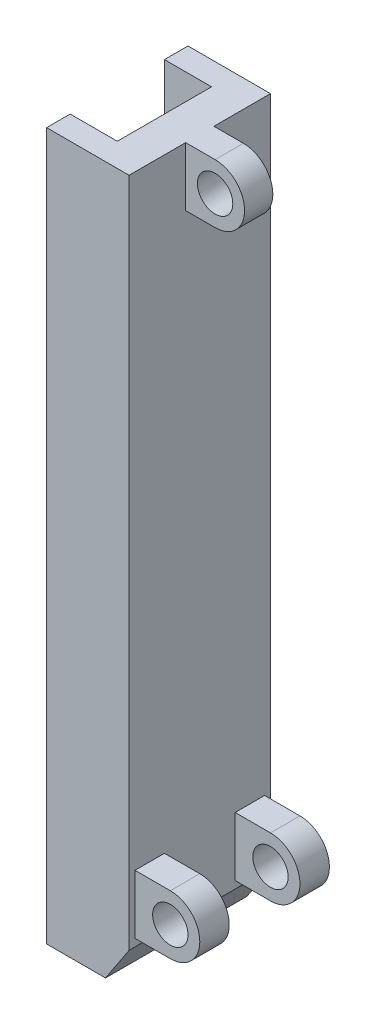
SolidWorks part; units mm, degrees
ref_plane "Front Plane" through (0, 0, 0) normal (0, 0, 1) x (1, 0, 0)
ref_plane "Top Plane" through (0, 0, 0) normal (0, 1, 0) x (1, 0, 0)
ref_plane "Right Plane" through (0, 0, 0) normal (1, 0, 0) x (0, 0, -1)
other "Configuration Table"
sketch "Sketch1" plane through (0, 0, 0) normal (0, 1, 0) x (1, 0, 0)
  line L0 (-20, 40) -> (-20, 60)
  line L1 (-20, 40) -> (20, 40)
  line L3 (-20, -40) -> (20, -40)
  line L4 (20, 40) -> (20, -40)
  line L5 (-20, 40) -> (20, -40) construction
  line L6 (-20, -40) -> (20, 40) construction
  line L7 (-20, 60) -> (50, 60)
  line L9 (-20, -60) -> (50, -60)
  line L10 (50, 60) -> (50, -60)
  line L11 (-50, 60) -> (50, -60) construction
  line L12 (-50, -60) -> (50, 60) construction
  line L13 (-20, -40) -> (-20, -60)
  point P0 (0, 0)
  point P6 (0, 0)
  dimension "D1" = 40
  dimension "D2" = 80
  dimension "D3" = 120
  dimension "D4" = 30
extrude "Boss-Extrude1" add sketch "Sketch1" along normal blind 600
sketch "Sketch2" plane through (0, 0, -60) normal (0, 0, -1) x (-1, 0, 0)
  line L0 (10.0315, 61.6536) -> (-80, 61.6536) construction
  line L1 (-34.9842, 36.6536) -> (-80, 36.6536)
  line L2 (-34.9842, 86.6536) -> (-80, 86.6536)
  line L3 (-50, 600) -> (-50, 0) construction
  line L4 (-34.9842, 86.6536) -> (-34.9842, 36.6536)
  arc A1 (-80, 86.6536) -> (-80, 36.6536) centre (-80, 61.6536) ccw
  circle A2 centre (-80, 61.6536) radius 15
  point P2 (-44.9842, 61.6536)
  dimension "D1" = 25
  dimension "D3" = 30
  dimension "D2" = 30
extrude "Boss-Extrude2" add sketch "Sketch2" against normal blind 30
mirror "Mirror1" about plane through (0, 0, 0) normal (0, 0, 1) of "Boss-Extrude2"
sketch "Sketch3" plane through (0, 0, 0) normal (0, 0, 1) x (1, 0, 0)
  line L0 (9.7473, 575) -> (75, 575) construction
  line L1 (42.3736, 600) -> (75, 600)
  line L2 (42.3736, 550) -> (75, 550)
  line L3 (50, 600) -> (50, 86.6536) construction
  line L4 (42.3736, 600) -> (42.3736, 550)
  line L5 (-20, 600) -> (50, 600) construction
  arc A1 (75, 550) -> (75, 600) centre (75, 575) ccw
  circle A2 centre (75, 575) radius 15
  point P2 (42.3736, 464.317)
  dimension "D1" = 25
  dimension "D3" = 30
  dimension "D2" = 25
extrude "Boss-Extrude3" add sketch "Sketch3" along normal blind 12 and the other way blind 12
sketch "Sketch4" plane through (0, 0, -60) normal (0, 0, -1) x (-1, 0, 0)
  line L1 (-50, 36.6536) -> (-114.9993, 36.6536)
  line L2 (-50, 36.6536) -> (-50, 91.6216)
  line L3 (-50, 91.6216) -> (-114.9993, 91.6216)
  line L4 (-114.9993, 36.6536) -> (-114.9993, 91.6216)
extrude "Cut-Extrude1" cut sketch "Sketch4" against normal blind 5
mirror "Mirror2" about plane through (0, 0, 0) normal (0, 0, 1) of "Cut-Extrude1"
sketch "Sketch5" plane through (0, 0, -60) normal (0, 0, -1) x (-1, 0, 0)
  line L0 (-50, 600) -> (-50, 0) construction
  line L1 (-50, 30.3406) -> (-30, 0)
  line L2 (66, 0) -> (-66, 0) construction
  line L3 (-30, 0) -> (-50, 0)
  line L4 (-50, 0) -> (-50, 30.3406)
  dimension "D1" = 20
extrude "Cut-Extrude2" cut sketch "Sketch5" against normal through all
